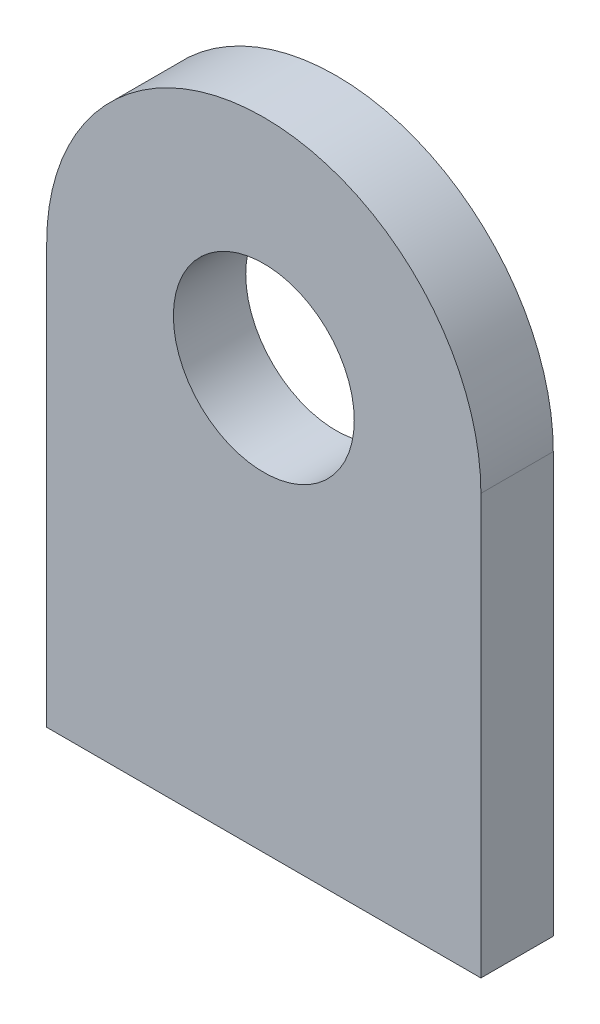
SolidWorks part; units mm, degrees
material "Q235"
ref_plane "Front Plane" through (0, 0, 0) normal (0, 0, 1) x (1, 0, 0)
ref_plane "Top Plane" through (0, 0, 0) normal (0, 1, 0) x (1, 0, 0)
ref_plane "Right Plane" through (0, 0, 0) normal (1, 0, 0) x (0, 0, -1)
sketch "Sketch1" plane through (0, 0, 0) normal (0, 0, 1) x (1, 0, 0)
  line L0 (0, 0) -> (0, 58)
  line L1 (60, 58) -> (60, 0)
  line L2 (60, 0) -> (0, 0)
  arc A0 (0, 58) -> (60, 58) centre (30, 58) cw
  circle A1 centre (30, 58) radius 12.5
  dimension "D3" = 25
  dimension "D1" = 60
  dimension "D2" = 58
extrude "Boss-Extrude1" add sketch "Sketch1" along normal blind 10
